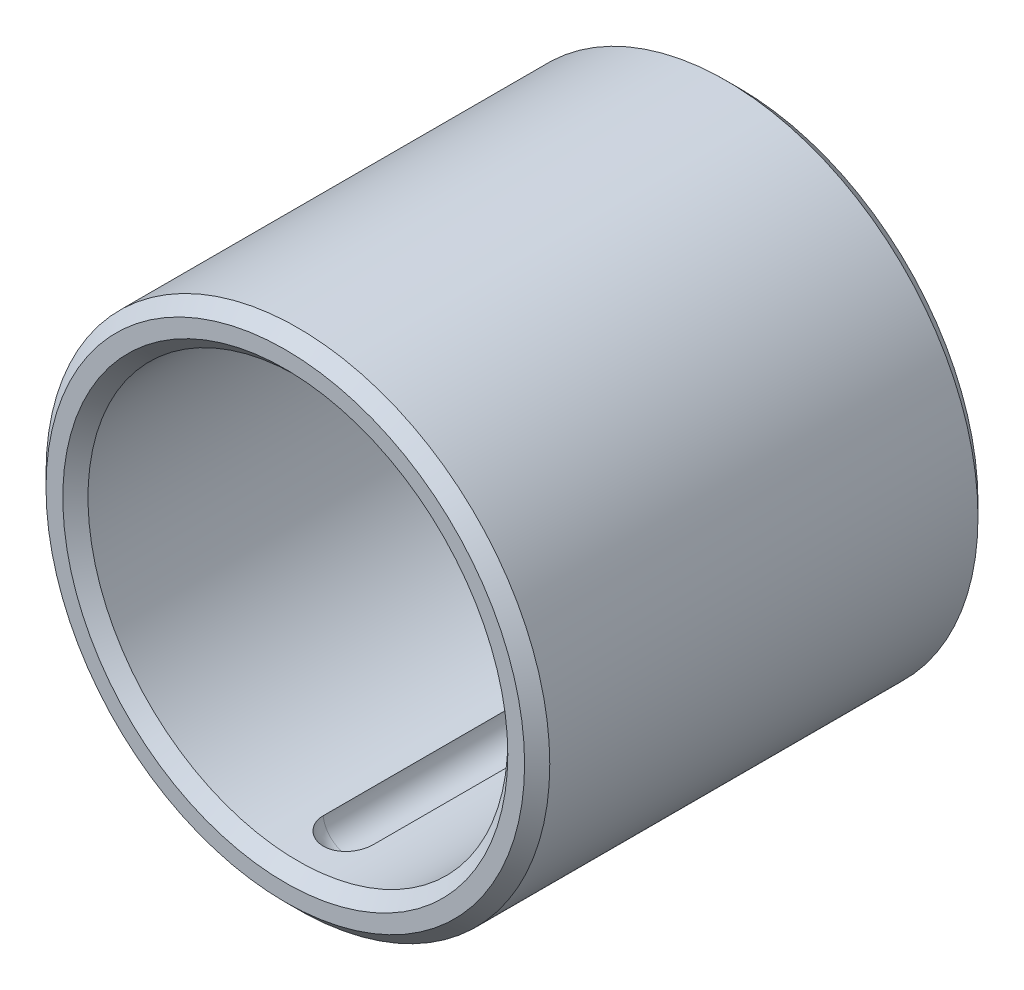
from build123d import *

# Parameters (mm, degrees)
SKETCH1_R           = 30
SKETCH1_R_2         = 25
BOSS_EXTRUDE1_DEPTH = 27
CHAMFER1_SIZE       = 1.5
CUT_EXTRUDE1_START  = -46.5
SKETCH2_R           = 3
CUT_EXTRUDE1_DEPTH  = 46.5


with BuildPart() as part:
    # Sketch1 → Boss-Extrude1 (new, symmetric)
    with BuildSketch(Plane.XY):
        Circle(SKETCH1_R)
        Circle(SKETCH1_R_2, mode=Mode.SUBTRACT)
    extrude(amount=BOSS_EXTRUDE1_DEPTH, both=True)

    # Chamfer1
    chamfer1_edges = [part.edges().sort_by_distance(p)[0] for p in [
        (-30, 0, -27),
        (-30, 0, 27),
        (-25, 0, -27),
        (-25, 0, 27),
    ]]
    chamfer(chamfer1_edges, length=CHAMFER1_SIZE)

    # Sketch3 → Cut-Revolve10 (revolve, cut)
    with BuildSketch(Plane(origin=(0, 0, 0), x_dir=(0, 0, -1), z_dir=(1, 0, 0))):
        with BuildLine():
            Line((-19.5, -21.5), (-19.5, -27.5))
            ThreePointArc((-19.5, -27.5), (-22.5, -24.5), (-19.5, -21.5))
        make_face()
    revolve(axis=Axis((0, -21.5, 19.5), (0, -1, 0)), mode=Mode.SUBTRACT)

    # Sketch2 → Cut-Extrude1 (cut)
    with BuildSketch(Plane(origin=(0, 0, -27), x_dir=(-1, 0, 0), z_dir=(0, 0, -1)).offset(CUT_EXTRUDE1_START)):
        with Locations((0, -24.5)):
            Circle(SKETCH2_R)
    extrude(amount=CUT_EXTRUDE1_DEPTH, mode=Mode.SUBTRACT)


solid = part.part
